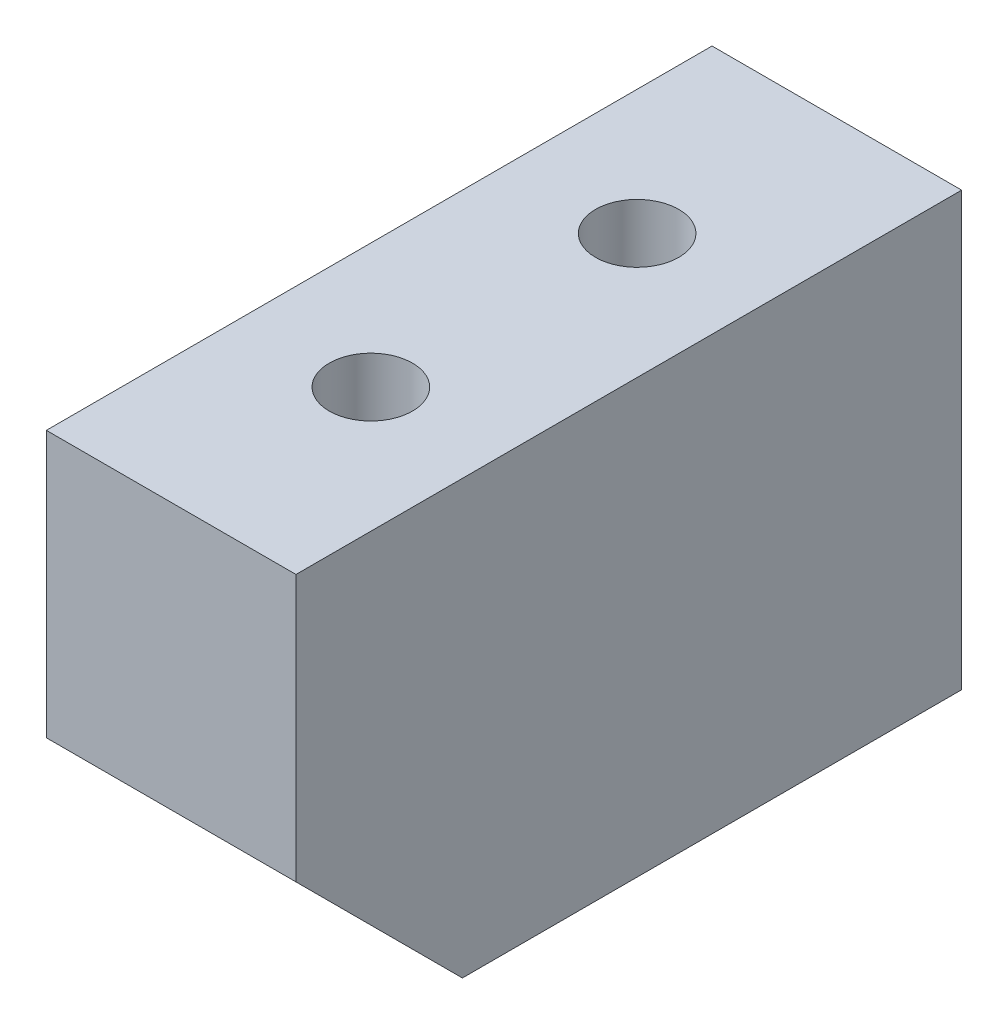
SolidWorks part; units mm, degrees
material "A6061"
ref_plane "前视基准面" through (0, 0, 0) normal (0, 0, 1) x (1, 0, 0)
ref_plane "上视基准面" through (0, 0, 0) normal (0, 1, 0) x (1, 0, 0)
ref_plane "右视基准面" through (0, 0, 0) normal (1, 0, 0) x (0, 0, -1)
sketch "草图1" plane through (0, 0, 0) normal (0, 0, 1) x (1, 0, 0)
  line L1 (-7.5, 13) -> (7.5, 13)
  line L2 (-7.5, 13) -> (-7.5, -13)
  line L3 (-7.5, -13) -> (7.5, -13)
  line L4 (7.5, 13) -> (7.5, -13)
  line L5 (-7.5, 13) -> (7.5, -13) construction
  line L6 (-7.5, -13) -> (7.5, 13) construction
  point P0 (0, 0)
  dimension "D1" = 26
  dimension "D2" = 15
extrude "凸台-拉伸1" add sketch "草图1" along normal blind 40
hole_wizard "M6 螺纹孔1" positions "草图3" profile "草图4" tap size "M6" standard "GB"
sketch "草图3" plane through (0, 13, 0) normal (0, 1, 0) x (1, 0, 0)
  line L0 (7.5, -40) -> (-7.5, -40) construction
  line L1 (0, -40) -> (0, -12) construction
  line L2 (7.5, 0) -> (-7.5, 0) construction
  point P0 (0, -12)
  point P10 (0, -28)
  dimension "D1" = 12
  dimension "D2" = 12
sketch "草图4" plane through (0, 13, 12) normal (1, 0, 0) x (0, 0, 1)
  line L0 (0, 0) -> (0, 16.5022)
  line L1 (0, 16.5022) -> (2.5, 15)
  line L2 (2.5, 15) -> (2.5, 0)
  line L5 (2.5, 0) -> (0, 0)
  line L10 (0, 16.5022) -> (-2.5, 15) construction
  line L11 (0, -6.35) -> (0, 107.95) construction
  dimension "螺纹孔钻头直径" = 5
  dimension "螺纹孔钻头深度" = 15
  dimension "导头角度" = 118
cosmetic thread "孔螺蚊线1"
cosmetic thread "孔螺蚊线3"
hole_wizard "M6 螺纹孔2" positions "草图5" profile "草图6" tap size "M6" standard "GB"
sketch "草图5" plane through (0, 0, 0) normal (0, 0, -1) x (-1, 0, 0)
  point P0 (0, 0)
sketch "草图6" plane through (0, 0, 0) normal (1, 0, 0) x (0, 1, 0)
  line L0 (0, 0) -> (0, 16.5022)
  line L1 (0, 16.5022) -> (2.5, 15)
  line L2 (2.5, 15) -> (2.5, 0)
  line L5 (2.5, 0) -> (0, 0)
  line L10 (0, 16.5022) -> (-2.5, 15) construction
  line L11 (0, -6.35) -> (0, 107.95) construction
  dimension "螺纹孔钻头直径" = 5
  dimension "螺纹孔钻头深度" = 15
  dimension "导头角度" = 118
cosmetic thread "孔螺蚊线2"
chamfer "倒角1" [suppressed] distance 2 angle 45
chamfer "倒角2" distance 10 angle 45 1 edges at (0, -13, 40)
